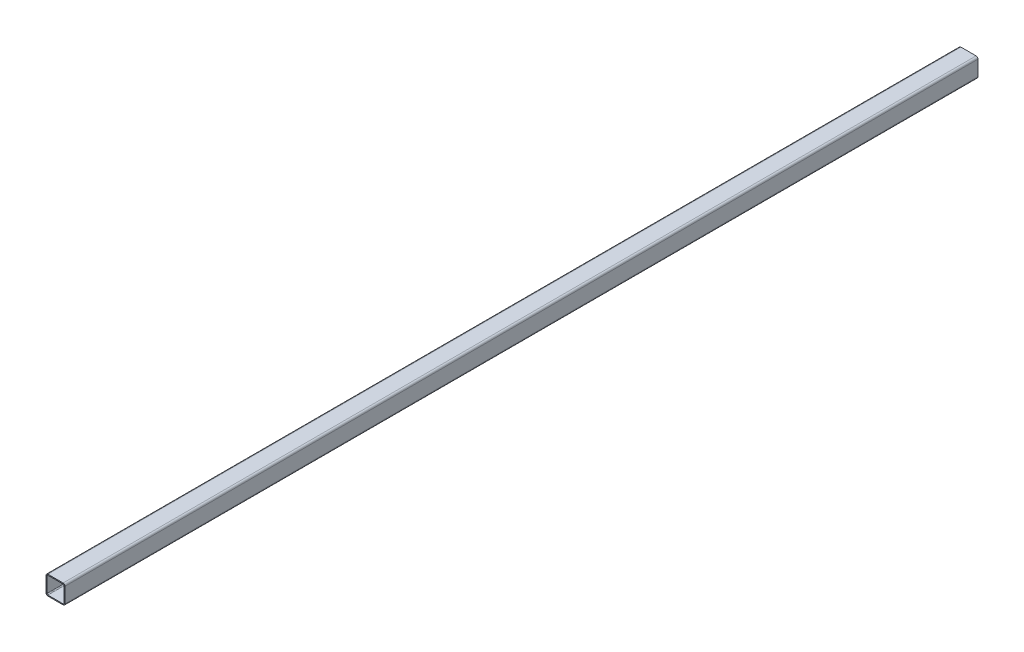
SolidWorks part; units mm, degrees
ref_plane "Front Plane" through (0, 0, 0) normal (0, 0, 1) x (1, 0, 0)
ref_plane "Top Plane" through (0, 0, 0) normal (0, 1, 0) x (1, 0, 0)
ref_plane "Right Plane" through (0, 0, 0) normal (1, 0, 0) x (0, 0, -1)
sketch "Sketch 1" plane through (0, 0, 0) normal (0, 0, 1) x (1, 0, 0)
  line L0 (0, 96.8978) -> (0, -107.4818) construction
  line L1 (-129.1971, 0) -> (137.9562, 0) construction
  line L2 (0, 50) -> (-40, 50)
  line L3 (-50, 40) -> (-50, 0)
  line L4 (0, 45) -> (-40, 45)
  line L5 (-45, 40) -> (-45, 0)
  line L6 (-45, -40) -> (-45, 0)
  line L7 (40, -45) -> (-40, -45)
  line L8 (-50, -40) -> (-50, 0)
  line L9 (40, -50) -> (-40, -50)
  line L10 (50, -40) -> (50, 0)
  line L11 (45, -40) -> (45, 0)
  line L12 (45, 40) -> (45, 0)
  line L13 (0, 45) -> (40, 45)
  line L14 (50, 40) -> (50, 0)
  line L15 (0, 50) -> (40, 50)
  arc A0 (-40, 50) -> (-50, 40) centre (-40, 40) ccw
  arc A1 (-40, 45) -> (-45, 40) centre (-40, 40) ccw
  arc A2 (-40, -45) -> (-45, -40) centre (-40, -40) cw
  arc A3 (-40, -50) -> (-50, -40) centre (-40, -40) cw
  arc A4 (40, -50) -> (50, -40) centre (40, -40) ccw
  arc A5 (40, -45) -> (45, -40) centre (40, -40) ccw
  arc A6 (40, 45) -> (45, 40) centre (40, 40) cw
  arc A7 (40, 50) -> (50, 40) centre (40, 40) cw
  point P34 (0, -50)
  point P35 (0, -45)
  dimension "D3" = 10
  dimension "D1" = 100
  dimension "D2" = 100
  dimension "D4" = 5
extrude "Boss-Extrude 1" add sketch "Sketch 1" along normal mid plane 4800
